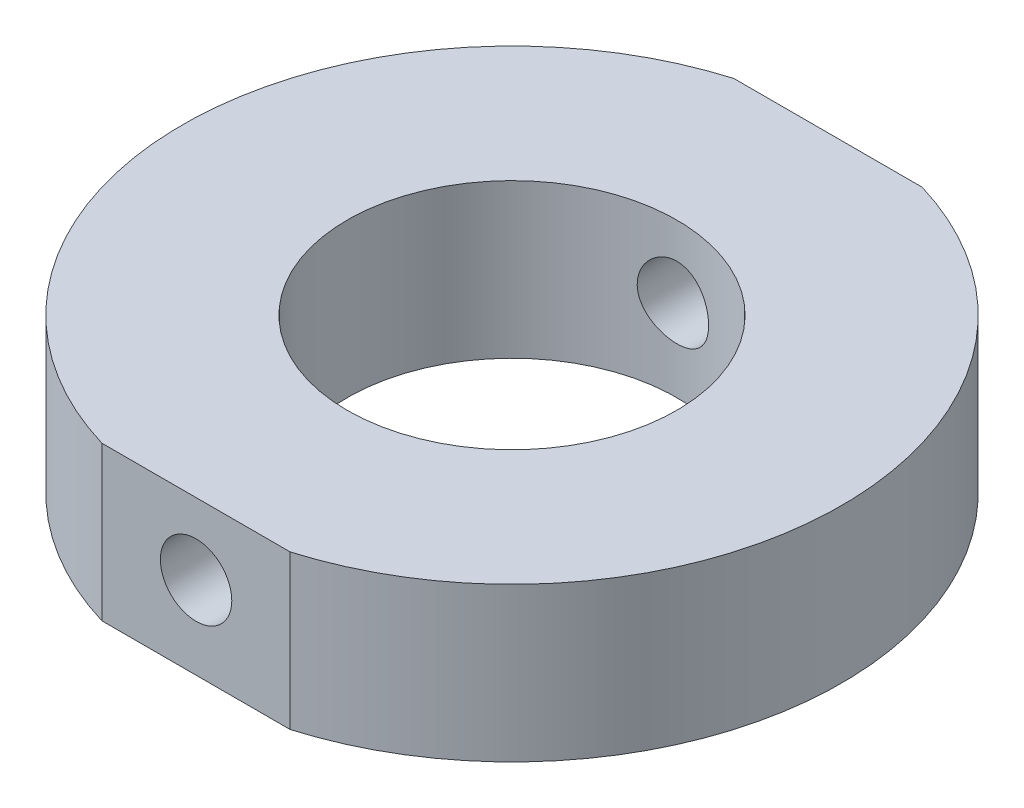
from build123d import *

# Parameters (mm, degrees)
SKETCH1_R               = 60
SKETCH1_R_2             = 30
BOSS_EXTRUDE1_DEPTH     = 14
CUT_EXTRUDE1_DEPTH      = 87
CUT_EXTRUDE1_DEPTH_BACK = 87
SKETCH2_OUTSIDE_W       = 156.4
SKETCH2_OUTSIDE_H       = 156.4
SKETCH2_OUTSIDE_W_2     = 160
SKETCH2_OUTSIDE_H_2     = 115
SKETCH3_R               = 6.5
CUT_EXTRUDE2_DEPTH      = 131.464554573


with BuildPart() as part:
    # Sketch1 → Boss-Extrude1 (new, symmetric)
    with BuildSketch(Plane(origin=(0, 0, 0), x_dir=(1, 0, 0), z_dir=(0, 1, 0))):
        with Locations(Location((0, 0, 0), (0, 0, 270))):
            Circle(SKETCH1_R)
        with Locations(Location((0, 0, 0), (0, 0, 270))):
            Circle(SKETCH1_R_2, mode=Mode.SUBTRACT)
    extrude(amount=BOSS_EXTRUDE1_DEPTH, both=True)

    # Sketch2 outside → Cut-Extrude1 (cut, two sides: drawn at the far end of the back side and taken through both)
    with BuildSketch(Plane(origin=(0, 0, 0), x_dir=(1, 0, 0), z_dir=(0, 1, 0)).offset(-CUT_EXTRUDE1_DEPTH_BACK)):
        Rectangle(SKETCH2_OUTSIDE_W, SKETCH2_OUTSIDE_H)
        Rectangle(SKETCH2_OUTSIDE_W_2, SKETCH2_OUTSIDE_H_2, mode=Mode.SUBTRACT)
    extrude(amount=CUT_EXTRUDE1_DEPTH + CUT_EXTRUDE1_DEPTH_BACK, mode=Mode.SUBTRACT)

    # Sketch3 → Cut-Extrude2 (cut, through all)
    with BuildSketch(Plane.XY.offset(57.5)):
        with Locations((0, 1)):
            Circle(SKETCH3_R)
    extrude(amount=-CUT_EXTRUDE2_DEPTH, mode=Mode.SUBTRACT)


solid = part.part
